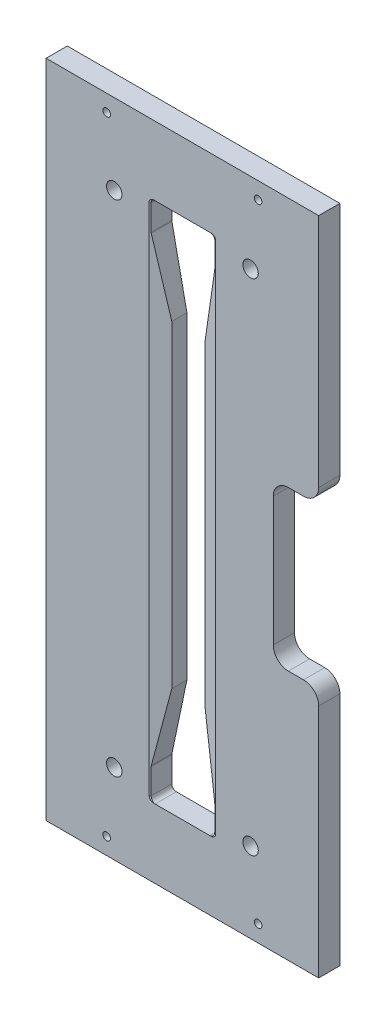
SolidWorks part; units mm, degrees
material "普通碳钢"
ref_plane "Front Plane" through (0, 0, 0) normal (0, 0, 1) x (1, 0, 0)
ref_plane "Top Plane" through (0, 0, 0) normal (0, 1, 0) x (1, 0, 0)
ref_plane "Right Plane" through (0, 0, 0) normal (1, 0, 0) x (0, 0, -1)
sketch "Sketch1" plane through (0, 0, 0) normal (0, 0, 1) x (1, 0, 0)
  line L0 (67, 45.5) -> (67, 390.5) construction
  line L1 (180, 436) -> (0, 436)
  line L2 (113, 390.5) -> (113, 45.5) construction
  line L3 (180, 0) -> (0, 0)
  line L4 (0, 436) -> (0, 0)
  line L5 (90, 390.5) -> (90, 45.5) construction
  line L6 (113, 390.5) -> (113, 45.5) construction
  line L7 (67, 390.5) -> (67, 45.5) construction
  line L8 (72, 45.5) -> (108, 45.5)
  line L9 (72, 390.5) -> (108, 390.5)
  line L10 (79, 323) -> (79, 113)
  line L11 (101, 113) -> (101, 323)
  line L12 (90, 218) -> (0, 218) construction
  line L13 (180, 436) -> (180, 0)
  line L14 (69.0644, 370.1943) -> (79, 323)
  line L15 (110.9356, 370.1943) -> (101, 323)
  line L16 (69, 48.5) -> (69, 65.1876)
  line L17 (69.0644, 65.8057) -> (79, 113)
  line L18 (69, 370.8124) -> (69, 387.5)
  line L19 (111, 370.8124) -> (111, 387.5)
  line L20 (111, 48.5) -> (111, 65.1876)
  line L21 (110.9356, 65.8057) -> (101, 113)
  arc A0 (113, 390.5) -> (67, 390.5) centre (90, 390.5) ccw construction
  arc A1 (67, 45.5) -> (113, 45.5) centre (90, 45.5) ccw construction
  arc A2 (110.9356, 370.1943) -> (111, 370.8124) centre (108, 370.8124) ccw
  arc A3 (69.0644, 370.1943) -> (69, 370.8124) centre (72, 370.8124) cw
  arc A4 (111, 387.5) -> (108, 390.5) centre (108, 387.5) ccw
  arc A5 (69, 387.5) -> (72, 390.5) centre (72, 387.5) cw
  arc A6 (111, 65.1876) -> (110.9356, 65.8057) centre (108, 65.1876) ccw
  arc A7 (69, 65.1876) -> (69.0644, 65.8057) centre (72, 65.1876) cw
  arc A8 (108, 45.5) -> (111, 48.5) centre (108, 48.5) ccw
  arc A9 (72, 45.5) -> (69, 48.5) centre (72, 48.5) cw
  point P9 (90, 218)
  point P29 (79, 218)
  point P32 (111, 370.5)
  point P35 (69, 370.5)
  point P41 (69, 390.5)
  point P44 (111, 65.5)
  point P47 (69, 65.5)
  point P52 (69, 45.5)
extrude "Boss-Extrude1" add sketch "Sketch1" against normal blind 14
sketch "Sketch5" plane through (0, 0, 0) normal (0, 0, 1) x (1, 0, 0)
  line L0 (150, 218) -> (180, 218) construction
  line L1 (150, 270.5) -> (180, 270.5)
  line L2 (150, 270.5) -> (150, 165.5)
  line L3 (150, 165.5) -> (180, 165.5)
  line L4 (180, 270.5) -> (180, 165.5)
  line L5 (180, 0) -> (180, 436) construction
  dimension "D1" = 105
  dimension "D2" = 30
extrude "Cut-Extrude1" cut sketch "Sketch5" against normal through all
hole_wizard "M12 Tapped Hole1" positions "Sketch9" profile "Sketch10" tap size "M12" standard "GB"
sketch "Sketch9" plane through (0, 0, -14) normal (0, 0, -1) x (-1, 0, 0)
  line L0 (-90, 390.5) -> (-90, 45.5) construction
  line L1 (-108, 390.5) -> (-72, 390.5) construction
  line L2 (-72, 45.5) -> (-108, 45.5) construction
  line L4 (-90, 218) -> (-79, 218) construction
  line L5 (-79, 323) -> (-79, 113) construction
  point P0 (-135, 383)
  point P2 (-45, 383)
  point P4 (-45, 53)
  point P6 (-135, 53)
  dimension "D1" = 90
  dimension "D2" = 330
sketch "Sketch10" plane through (135, 383, -14) normal (1, 0, 0) x (0, 1, 0)
  line L0 (0, 0) -> (0, 35.8144)
  line L1 (0, 35.8144) -> (5.1, 32.75)
  line L2 (5.1, 32.75) -> (5.1, 0)
  line L5 (5.1, 0) -> (0, 0)
  line L10 (0, 35.8144) -> (-5.1, 32.75) construction
  line L11 (0, -6.35) -> (0, 107.95) construction
  dimension "螺纹孔钻头直径" = 10.2
  dimension "螺纹孔钻头深度" = 32.75
  dimension "导头角度" = 118
cosmetic thread "Cosmetic Thread9" parameters "D1"=14, "D2"=12
cosmetic thread "Cosmetic Thread10" parameters "D1"=14, "D2"=12
cosmetic thread "Cosmetic Thread11" parameters "D1"=14, "D2"=12
cosmetic thread "Cosmetic Thread12" parameters "D1"=14, "D2"=12
fillet "Fillet1" radius 10 4 edges at (180, 165.5, -7) (150, 165.5, -7) (150, 270.5, -7) (180, 270.5, -7)
hole_wizard "M6 Tapped Hole1" positions "Sketch6" profile "Sketch7" tap size "M6" standard "GB"
sketch "Sketch6" plane through (0, 0, 0) normal (0, 0, 1) x (1, 0, 0)
  line L0 (90, 390.5) -> (90, 45.5) construction
  line L2 (101, 218) -> (150, 218) construction
  line L4 (150, 260.5) -> (150, 175.5) construction
  line L5 (101, 113) -> (101, 323) construction
  line L6 (108, 390.5) -> (72, 390.5) construction
  line L7 (108, 390.5) -> (72, 390.5) construction
  line L8 (72, 45.5) -> (108, 45.5) construction
  point P0 (40, 425)
  point P2 (140, 425)
  point P4 (40, 11)
  point P6 (140, 11)
  point P26 (90, 390.5)
  dimension "D1" = 100
  dimension "D2" = 414
sketch "Sketch7" plane through (40, 425, 0) normal (1, 0, 0) x (0, -1, 0)
  line L0 (0, 0) -> (0, 18.5022)
  line L1 (0, 18.5022) -> (2.5, 17)
  line L2 (2.5, 17) -> (2.5, 0)
  line L5 (2.5, 0) -> (0, 0)
  line L10 (0, 18.5022) -> (-2.5, 17) construction
  line L11 (0, -6.35) -> (0, 107.95) construction
  dimension "螺纹孔钻头直径" = 5
  dimension "螺纹孔钻头深度" = 17
  dimension "导头角度" = 118
cosmetic thread "Cosmetic Thread5" parameters "D1"=12, "D2"=6
cosmetic thread "Cosmetic Thread6" parameters "D1"=12, "D2"=6
cosmetic thread "Cosmetic Thread7" parameters "D1"=12, "D2"=6
cosmetic thread "Cosmetic Thread8" parameters "D1"=12, "D2"=6
sketch "Sketch8" plane through (0, 0, 0) normal (0, 0, 1) x (1, 0, 0)
  line L0 (90, 390.5) -> (90, 45.5) construction
  line L1 (108, 390.5) -> (72, 390.5) construction
  line L2 (72, 45.5) -> (108, 45.5) construction
  line L3 (71, 390.5) -> (109, 390.5)
  line L4 (68, 387.5) -> (68, 48.5)
  line L5 (71, 45.5) -> (109, 45.5)
  line L6 (112, 387.5) -> (112, 48.5)
  line L7 (68, 390.5) -> (112, 45.5) construction
  line L8 (68, 45.5) -> (112, 390.5) construction
  arc A0 (112, 387.5) -> (109, 390.5) centre (109, 387.5) ccw
  arc A1 (68, 387.5) -> (71, 390.5) centre (71, 387.5) cw
  arc A2 (109, 45.5) -> (112, 48.5) centre (109, 48.5) ccw
  arc A3 (68, 48.5) -> (71, 45.5) centre (71, 48.5) ccw
  point P8 (90, 218)
  point P9 (90, 218)
  dimension "D1" = 3
  dimension "D2" = 44
extrude "Cut-Extrude2" cut sketch "Sketch8" against normal blind 5 draft 70
equation "\"D7@Sketch1\"=\"D6@Sketch1\""
